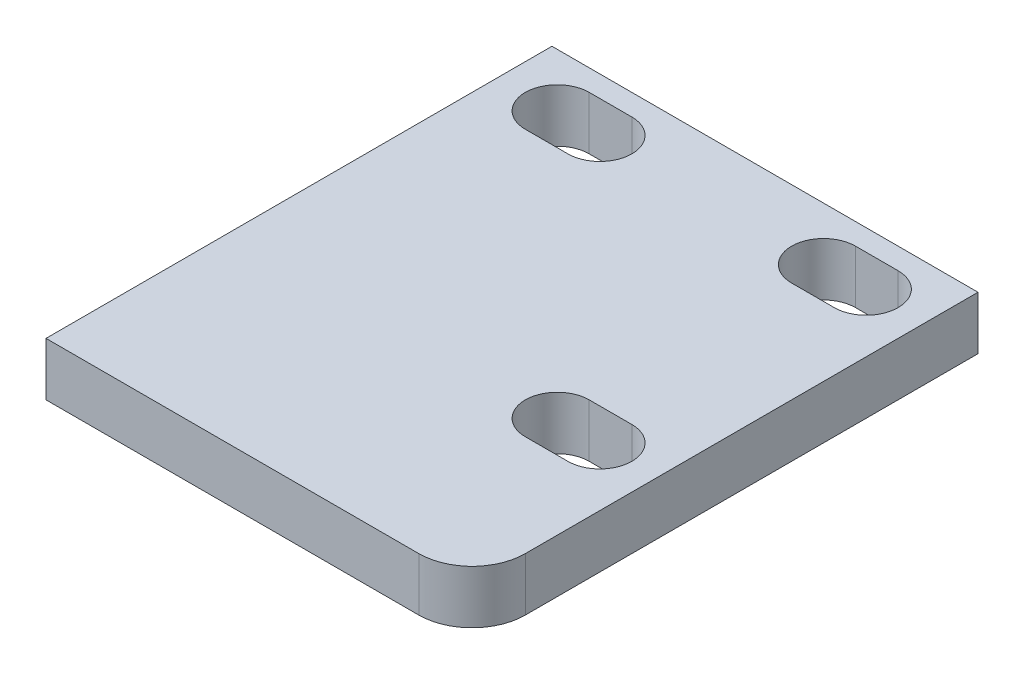
from build123d import *

# Parameters (mm, degrees)
BOSS_EXTRUDE1_DEPTH = 10


with BuildPart() as part:
    # Sketch1 → Boss-Extrude1 (new body)
    with BuildSketch(Plane(origin=(0, 0, 0), x_dir=(1, 0, 0), z_dir=(0, 1, 0))):
        with BuildLine():
            Line((-40, -47.5), (30, -47.5))
            ThreePointArc((30, -47.5), (37.071067812, -44.571067812), (40, -37.5))
            Line((40, -37.5), (40, 47.5))
            Line((40, 47.5), (-40, 47.5))
            Line((-40, 47.5), (-40, -47.5))
        make_face()
        with BuildLine():
            Line((-29, 43.5), (-21, 43.5))
            ThreePointArc((-21, 43.5), (-15, 37.5), (-21, 31.5))
            Line((-21, 31.5), (-29, 31.5))
            ThreePointArc((-29, 31.5), (-35, 37.5), (-29, 43.5))
        make_face(mode=Mode.SUBTRACT)
        with BuildLine():
            Line((21, 31.5), (29, 31.5))
            ThreePointArc((29, 31.5), (35, 37.5), (29, 43.5))
            Line((29, 43.5), (21, 43.5))
            ThreePointArc((21, 43.5), (15, 37.5), (21, 31.5))
        make_face(mode=Mode.SUBTRACT)
        with BuildLine():
            Line((21, -18.5), (29, -18.5))
            ThreePointArc((29, -18.5), (35, -12.5), (29, -6.5))
            Line((29, -6.5), (21, -6.5))
            ThreePointArc((21, -6.5), (15, -12.5), (21, -18.5))
        make_face(mode=Mode.SUBTRACT)
    extrude(amount=BOSS_EXTRUDE1_DEPTH)


solid = part.part
